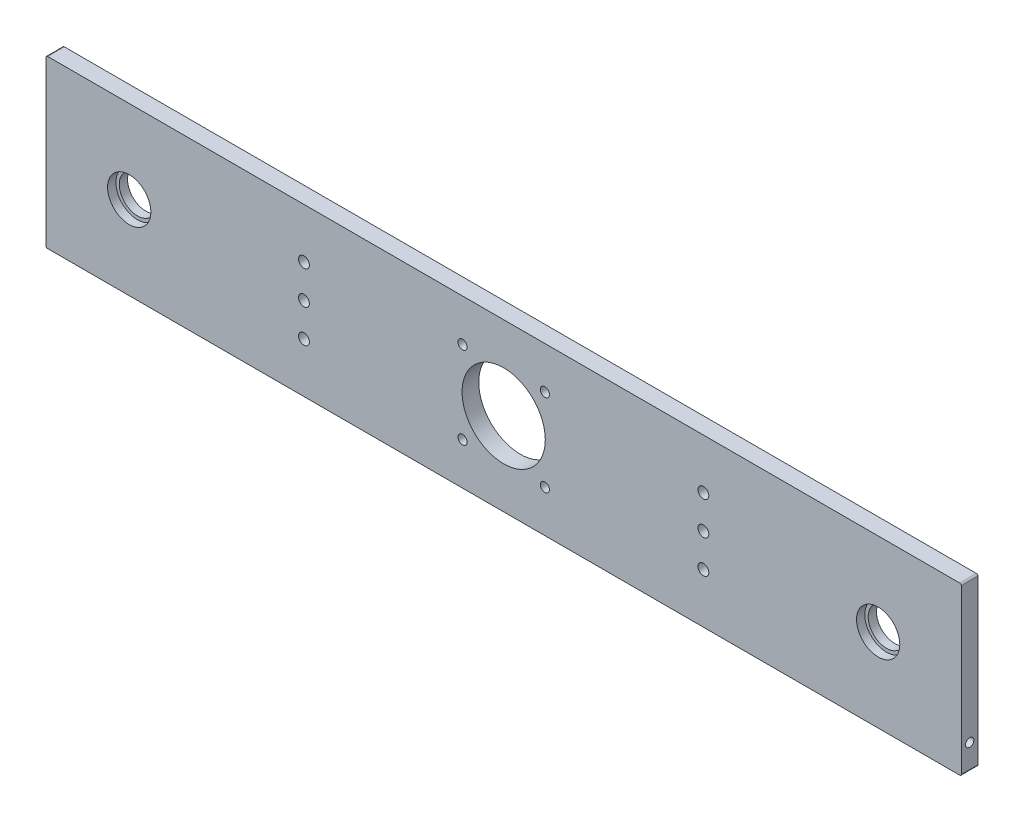
SolidWorks part; units mm, degrees
material "6061-T6 "
ref_plane "Front Plane" through (0, 0, 0) normal (0, 0, 1) x (1, 0, 0)
ref_plane "Top Plane" through (0, 0, 0) normal (0, 1, 0) x (1, 0, 0)
ref_plane "Right Plane" through (0, 0, 0) normal (1, 0, 0) x (0, 0, -1)
sketch "Sketch1" plane through (0, 0, 0) normal (0, 0, 1) x (1, 0, 0)
  line L1 (275, -50) -> (-275, -50)
  line L2 (275, -50) -> (275, 50)
  line L3 (275, 50) -> (-275, 50)
  line L4 (-275, -50) -> (-275, 50)
  line L5 (275, -50) -> (-275, 50) construction
  line L6 (275, 50) -> (-275, -50) construction
  point P0 (0, 0)
  dimension "D1" = 100
  dimension "D2" = 550
extrude "Boss-Extrude1" add sketch "Sketch1" along normal blind 10
sketch "Sketch3" plane through (0, 0, 10) normal (0, 0, 1) x (1, 0, 0)
  line L0 (0, 50) -> (0, -50) construction
  line L1 (275, 50) -> (-275, 50) construction
  line L2 (-275, -50) -> (275, -50) construction
  circle A0 centre (225, 0) radius 13
  circle A1 centre (-225, 0) radius 13
  dimension "D1" = 26
  dimension "D2" = 225
extrude "Cut-Extrude2" cut sketch "Sketch3" against normal blind 5
sketch "Sketch4" plane through (0, 0, 5) normal (0, 0, 1) x (1, 0, 0)
  line L0 (0, 50) -> (0, -50) construction
  line L1 (275, 50) -> (-275, 50) construction
  line L2 (-275, -50) -> (275, -50) construction
  circle A0 centre (225, 0) radius 11
  circle A1 centre (-225, 0) radius 11
  dimension "D1" = 22
extrude "Cut-Extrude3" cut sketch "Sketch4" against normal through all
sketch "Sketch5" plane through (0, 0, 10) normal (0, 0, 1) x (1, 0, 0)
  circle A0 centre (0, 0) radius 25
  dimension "D1" = 50
extrude "Cut-Extrude4" cut sketch "Sketch5" against normal through all
sketch "Sketch6" plane through (0, 0, 10) normal (0, 0, 1) x (1, 0, 0)
  line L0 (-24.7487, 24.7487) -> (24.7487, -24.7487) construction
  line L1 (-24.7487, -24.7487) -> (24.7487, 24.7487) construction
  line L2 (0, 0) -> (35, 0) construction
  circle A0 centre (0, 0) radius 35 construction
  circle A1 centre (-24.7487, 24.7487) radius 2.75
  circle A2 centre (24.7487, 24.7487) radius 2.75
  circle A3 centre (24.7487, -24.7487) radius 2.75
  circle A4 centre (-24.7487, -24.7487) radius 2.75
  dimension "D1" = 70
  dimension "D4" = 5.5
  dimension "D2" = 45
  dimension "D3" = 90
extrude "Cut-Extrude5" cut sketch "Sketch6" against normal through all
sketch "Sketch7" plane through (0, 0, 10) normal (0, 0, 1) x (1, 0, 0)
  line L0 (0, 50) -> (0, -50) construction
  line L1 (275, 50) -> (-275, 50) construction
  line L2 (-275, -50) -> (275, -50) construction
  line L3 (-275, 0) -> (275, 0) construction
  line L4 (-275, 50) -> (-275, -50) construction
  line L5 (275, -50) -> (275, 50) construction
  circle A2 centre (-120, -20) radius 3.25
  circle A3 centre (120, -20) radius 3.25
  circle A4 centre (120, 20) radius 3.25
  circle A5 centre (-120, 20) radius 3.25
  circle A6 centre (-120, 0) radius 3.25
  circle A7 centre (120, 0) radius 3.25
  dimension "D2" = 20
  dimension "D1" = 240
  dimension "D3" = 6.5
extrude "Cut-Extrude6" cut sketch "Sketch7" against normal through all
fillet "Fillet1" radius 1 4 edges at (-275, -50, 5) (-275, 50, 5) (275, -50, 5) (275, 50, 5)
hole_wizard "M6 Tapped Hole1" positions "Sketch8" profile "Sketch9" tap size "M6" standard "GB"
sketch "Sketch8" plane through (-275, 0, 0) normal (-1, 0, 0) x (0, 0, 1)
  line L0 (10, 49) -> (0, 49) construction
  line L1 (10, -50) -> (0, -50) construction
  point P0 (5, -35)
  point P7 (5, 49)
  dimension "D1" = 15
sketch "Sketch9" plane through (-275, -35, 5) normal (0, 1, 0) x (0, 0, 1)
  line L0 (0, 0) -> (0, 19.5022)
  line L1 (0, 19.5022) -> (2.5, 18)
  line L2 (2.5, 18) -> (2.5, 0)
  line L5 (2.5, 0) -> (0, 0)
  line L10 (0, 19.5022) -> (-2.5, 18) construction
  line L11 (0, -6.35) -> (0, 107.95) construction
  dimension "螺纹孔钻头直径" = 5
  dimension "螺纹孔钻头深度" = 18
  dimension "导头角度" = 118
cosmetic thread "Hole thread1" parameters "D1"=15, "D2"=6
mirror "Mirror1" about plane through (0, 0, 0) normal (1, 0, 0) of "M6 Tapped Hole1"
